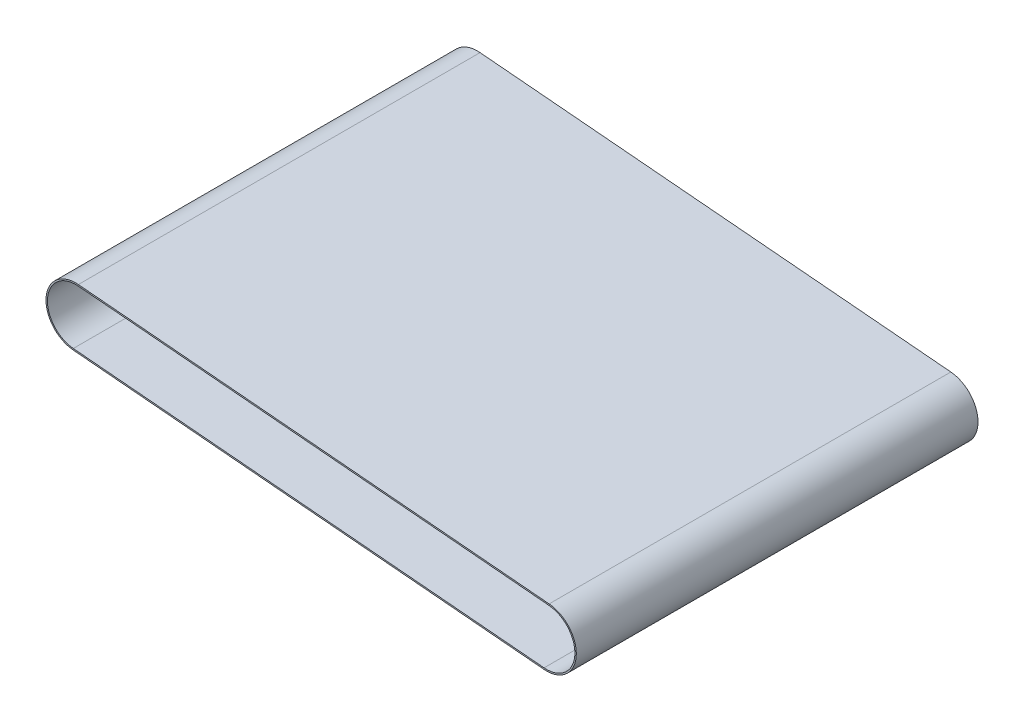
SolidWorks part; units mm, degrees
ref_plane "前视基准面" through (0, 0, 0) normal (0, 0, 1) x (1, 0, 0)
ref_plane "上视基准面" through (0, 0, 0) normal (0, 1, 0) x (1, 0, 0)
ref_plane "右视基准面" through (0, 0, 0) normal (1, 0, 0) x (0, 0, -1)
sketch "草图1" plane through (0, 0, 425) normal (0, 0, 1) x (1, 0, 0)
  line L0 (2514.6954, 796.0952) -> (3510.8901, 708.9394) construction
  line L1 (2519.9247, 855.8669) -> (3516.1194, 768.7111)
  line L2 (2509.466, 736.3235) -> (3505.6607, 649.1678)
  line L3 (2520.1862, 858.8555) -> (3516.3809, 771.6997)
  line L4 (2509.2046, 733.3349) -> (3505.3993, 646.1792)
  line L5 (2514.6954, 796.0952) -> (3510.8901, 708.9394) construction
  arc A0 (2519.9247, 855.8669) -> (2509.466, 736.3235) centre (2514.6954, 796.0952) ccw
  arc A1 (3505.6607, 649.1678) -> (3516.1194, 768.7111) centre (3510.8901, 708.9394) ccw
  arc A3 (3505.3993, 646.1792) -> (3516.3809, 771.6997) centre (3510.8901, 708.9394) ccw
  arc A4 (2520.1862, 858.8555) -> (2509.2046, 733.3349) centre (2514.6954, 796.0952) ccw
  circle A5 centre (3510.8901, 708.9394) radius 60 construction
  circle A7 centre (2514.6954, 796.0952) radius 60 construction
  point P4 (3012.7927, 752.5173)
  dimension "D1" = 3
extrude "凸台-拉伸1" add sketch "草图1" against normal up to surface (850 mm away)
